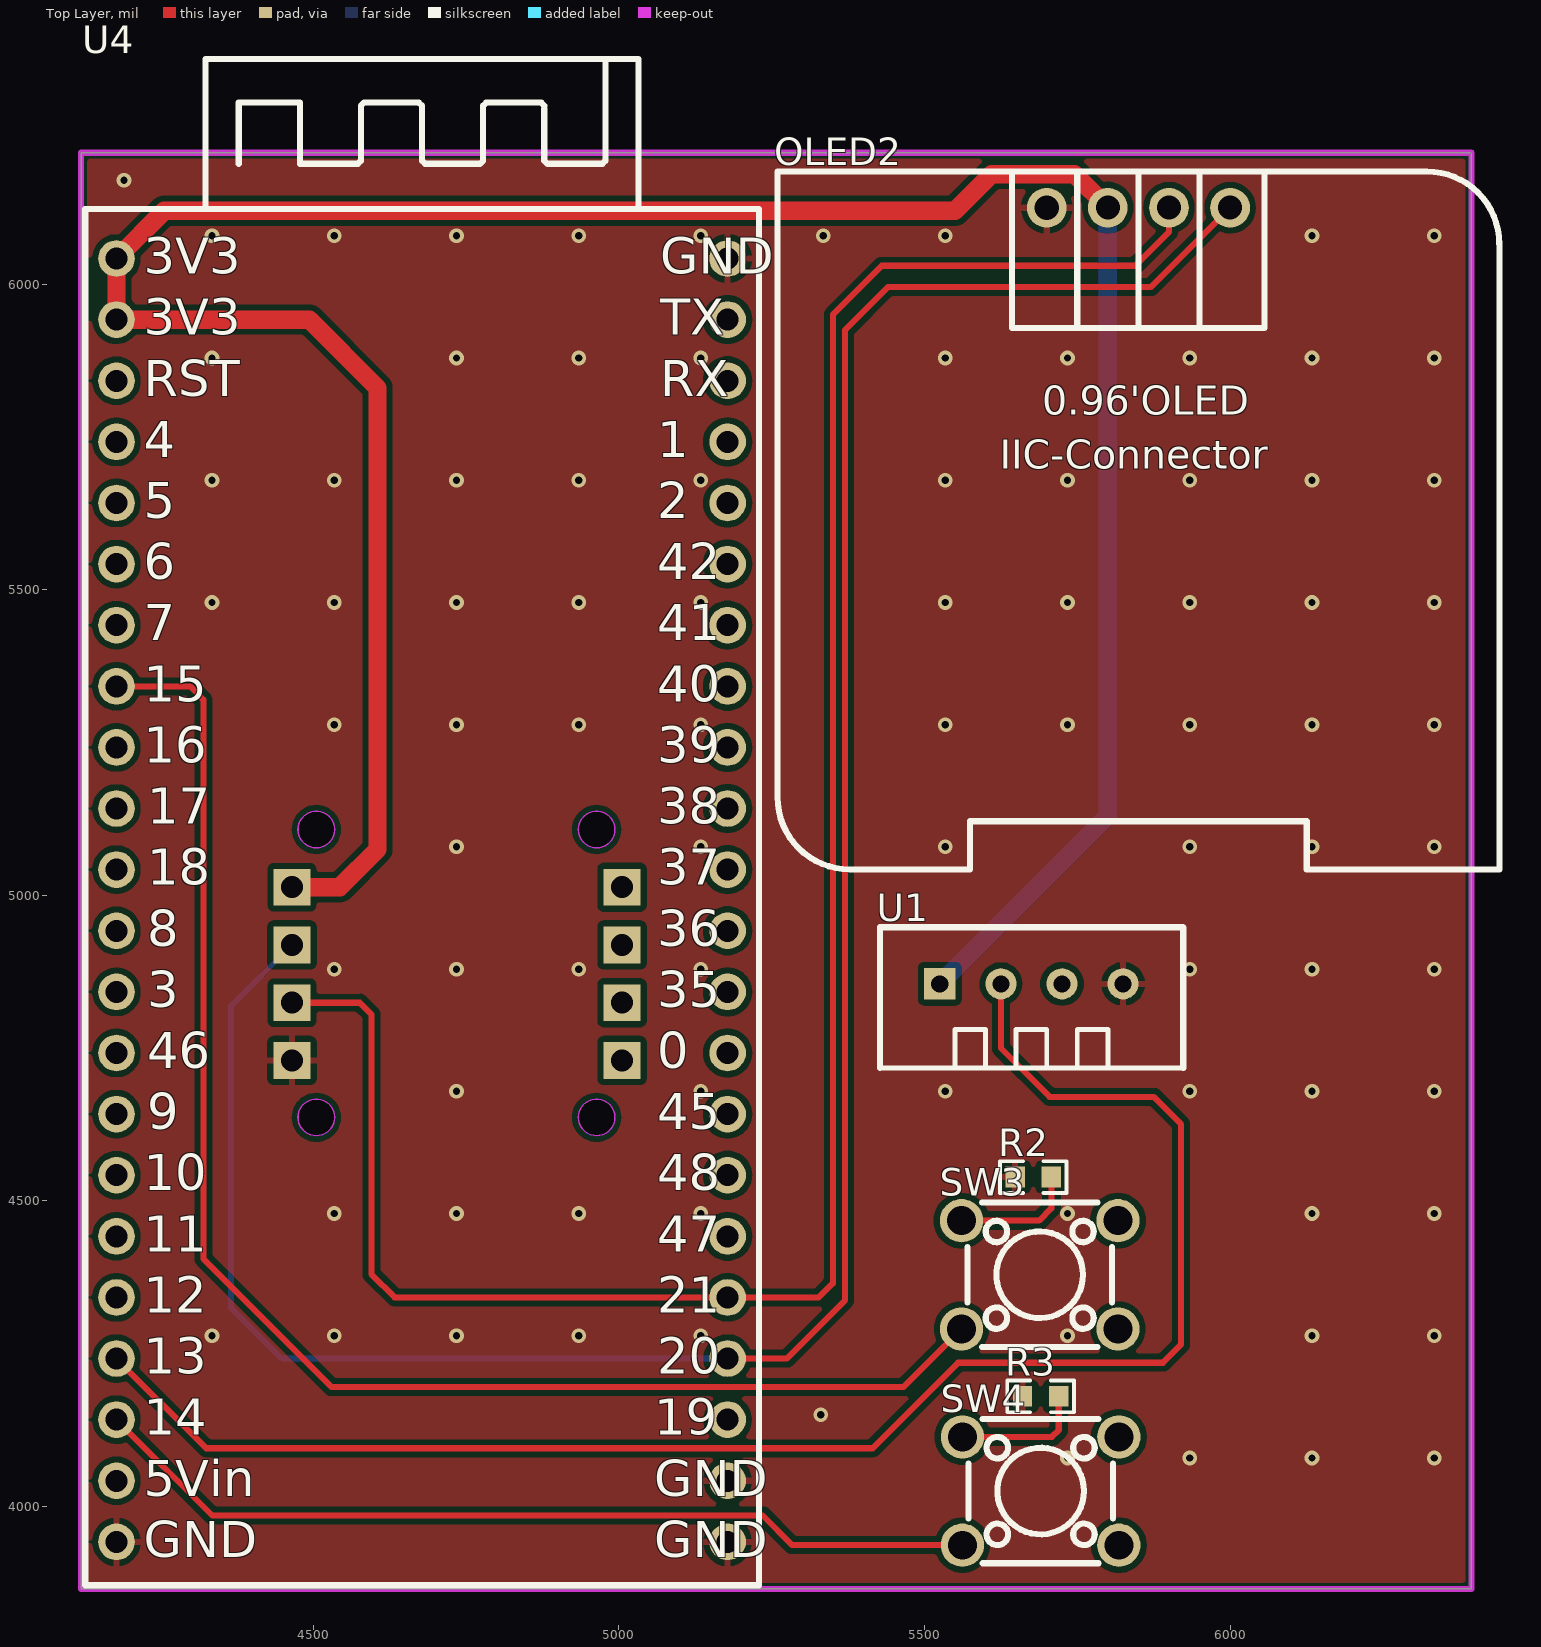
[diagram p0: Top Layer view]
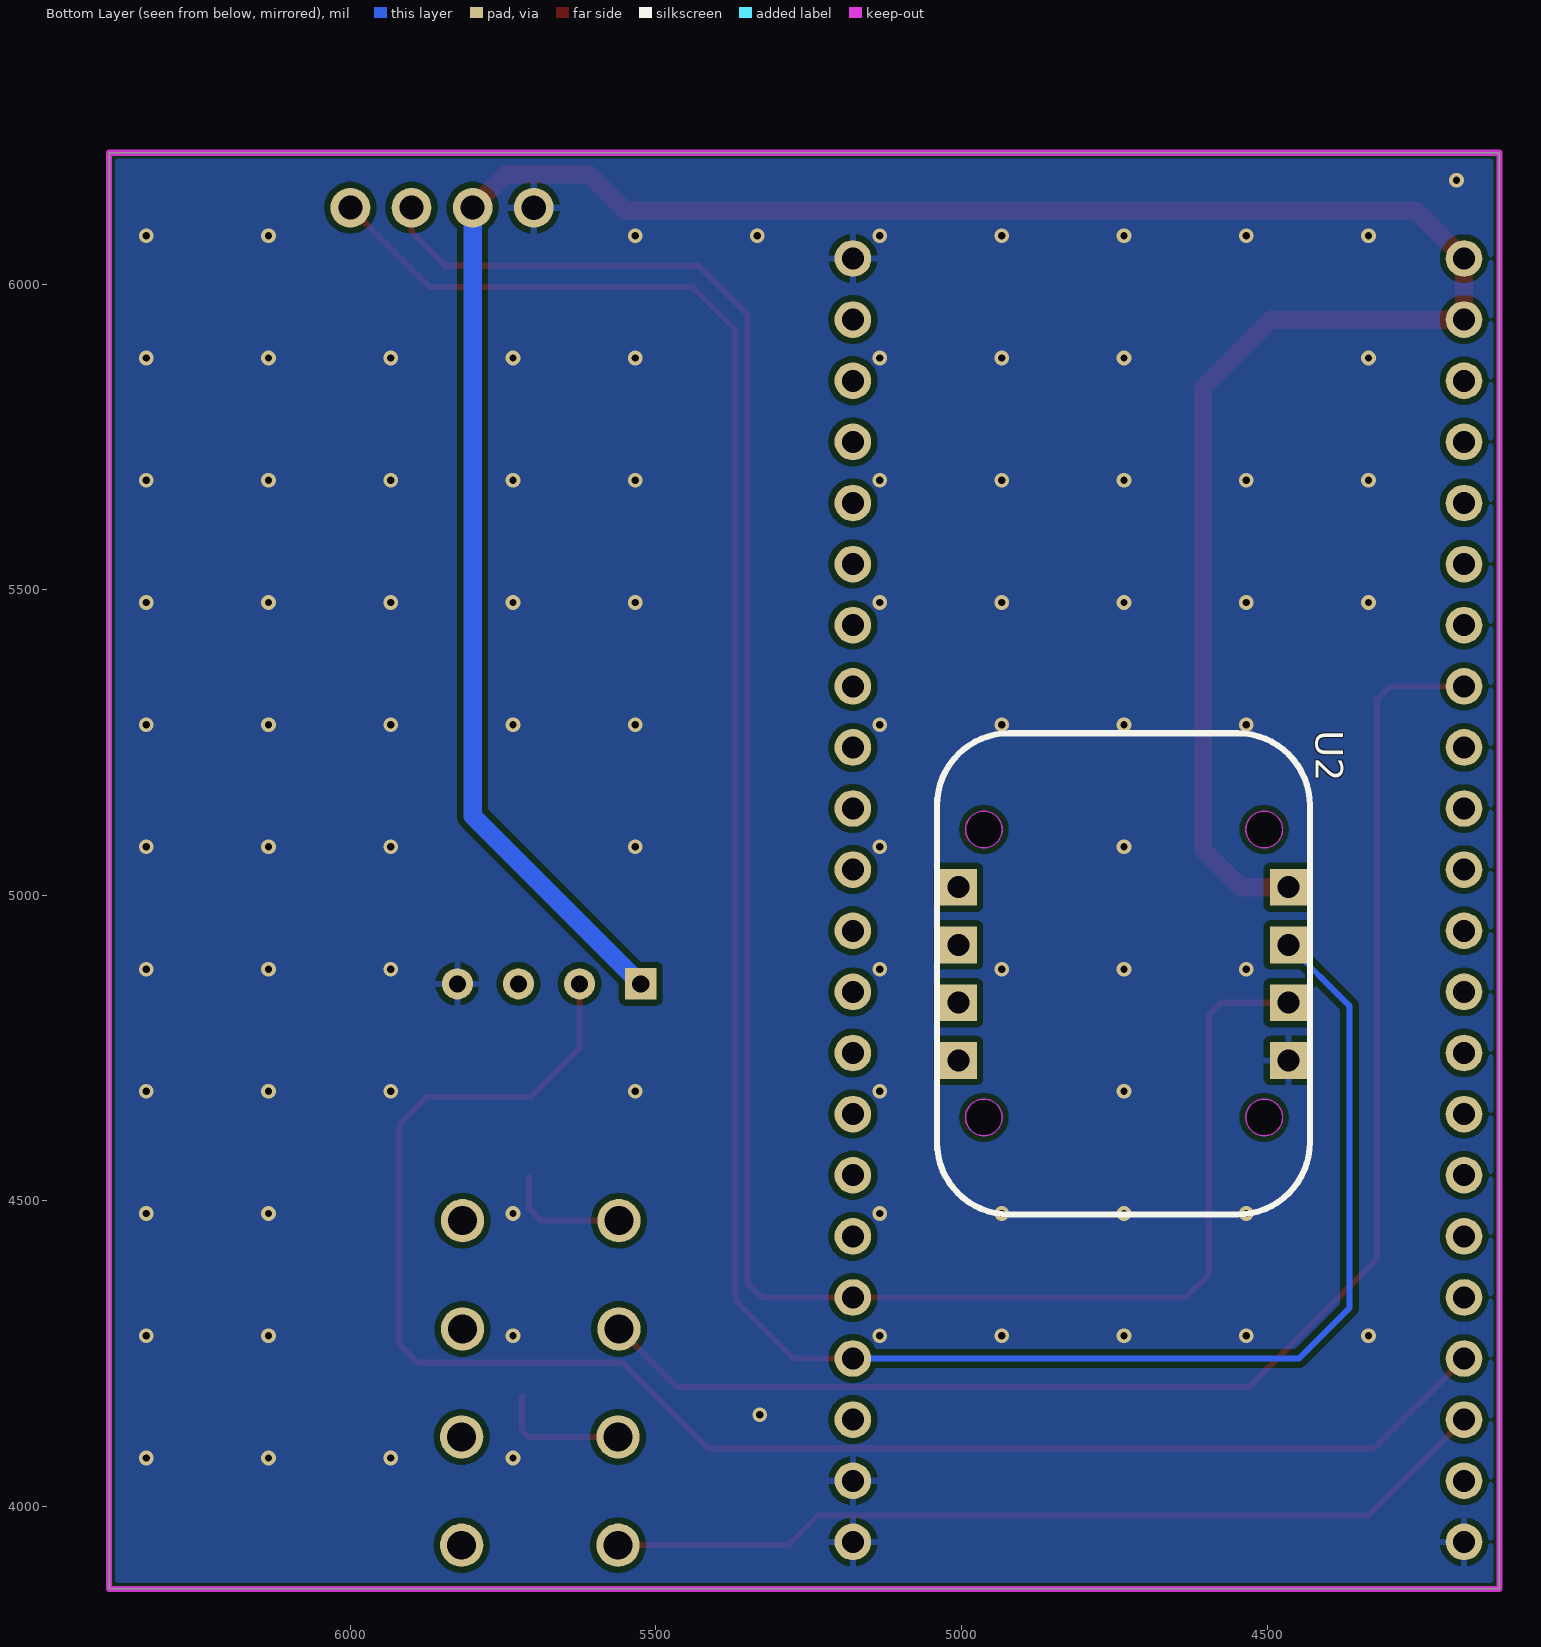
[diagram p1: Bottom Layer view, seen from below]
# Altium PCB MISC61243.pcbdoc
Units mil, origin at the board's own origin, x right, y up, seen from the top; angles counter-clockwise.
Board outline 2275 x 2350 mil, 2 copper layers (Top Layer, Bottom Layer), stack 62.206 mil thick; 8 components, 43 nets, 72 pads, 87 vias.

## Layer stack, top to bottom
Top Solder Mask Layer: solder mask 0.394, Dk 3.3
Top Layer: signal copper 1.379
Dielectric1: surface 59.449, FR4, Dk 4.5
Bottom Layer: signal copper 1.378
Bottom Solder Mask Layer: solder mask 0.394, Dk 3.3

## Board outline
4120,6215 4120,3865 6395,3865 6395,6215

## Design rules (kind name [scope] priority, off if disabled: settings)
BoardOutlineClearance copperThickness2oz_1 [All] p2 off: genericclearance=7.99 ignorepadtopadclearanceinfootprint=FALSE except(0: Arc-SplitContinuation Track-SplitContinuation SMDPad-SplitContinuation THPad-SplitContinuation Via-SplitContinuation Fill-SplitContinuation Region-SplitContinuation Poly-SplitContinuation Text-SplitContinuation Hole-SplitContinuation; 5.98: Arc-CutoutEdge Track-CutoutEdge SMDPad-CutoutEdge THPad-CutoutEdge Via-CutoutEdge Text-CutoutEdge; 6.9: Hole-OutlineEdge Hole-CutoutEdge; 10: Poly-OutlineEdge Poly-CutoutEdge; 11.81: Arc-OutlineEdge Track-OutlineEdge SMDPad-OutlineEdge THPad-OutlineEdge Via-OutlineEdge Fill-OutlineEdge Region-OutlineEdge Text-OutlineEdge Fill-CutoutEdge Region-CutoutEdge)
BoardOutlineClearance Plane_innerPlane_1 [All] p4 off: genericclearance=4.02 ignorepadtopadclearanceinfootprint=FALSE except(0: Arc-SplitContinuation Track-SplitContinuation SMDPad-SplitContinuation THPad-SplitContinuation Via-SplitContinuation Fill-SplitContinuation Region-SplitContinuation Poly-SplitContinuation Text-SplitContinuation Hole-SplitContinuation; 5.98: Arc-CutoutEdge Track-CutoutEdge SMDPad-CutoutEdge THPad-CutoutEdge Via-CutoutEdge Text-CutoutEdge; 6.9: Hole-OutlineEdge Hole-CutoutEdge; 10: Poly-OutlineEdge Poly-CutoutEdge; 11.81: Arc-OutlineEdge Track-OutlineEdge SMDPad-OutlineEdge THPad-OutlineEdge Via-OutlineEdge Fill-OutlineEdge Region-OutlineEdge Text-OutlineEdge Fill-CutoutEdge Region-CutoutEdge)
BoardOutlineClearance Copper_copperRegion_1 [All] p6 off: genericclearance=4.02 ignorepadtopadclearanceinfootprint=FALSE except(0: Arc-SplitContinuation Track-SplitContinuation SMDPad-SplitContinuation THPad-SplitContinuation Via-SplitContinuation Fill-SplitContinuation Region-SplitContinuation Poly-SplitContinuation Text-SplitContinuation Hole-SplitContinuation; 5.98: Arc-CutoutEdge Track-CutoutEdge SMDPad-CutoutEdge THPad-CutoutEdge Via-CutoutEdge Text-CutoutEdge; 6.9: Hole-OutlineEdge Hole-CutoutEdge; 10: Poly-OutlineEdge Poly-CutoutEdge; 11.81: Arc-OutlineEdge Track-OutlineEdge SMDPad-OutlineEdge THPad-OutlineEdge Via-OutlineEdge Fill-OutlineEdge Region-OutlineEdge Text-OutlineEdge Fill-CutoutEdge Region-CutoutEdge)
BoardOutlineClearance Copper_copperRegion_copperThickness1oz_1 [All] p8 off: genericclearance=4.02 ignorepadtopadclearanceinfootprint=FALSE except(0: Arc-SplitContinuation Track-SplitContinuation SMDPad-SplitContinuation THPad-SplitContinuation Via-SplitContinuation Fill-SplitContinuation Region-SplitContinuation Poly-SplitContinuation Text-SplitContinuation Hole-SplitContinuation; 5.98: Arc-CutoutEdge Track-CutoutEdge SMDPad-CutoutEdge THPad-CutoutEdge Via-CutoutEdge Text-CutoutEdge; 6.9: Hole-OutlineEdge Hole-CutoutEdge; 10: Poly-OutlineEdge Poly-CutoutEdge; 11.81: Arc-OutlineEdge Track-OutlineEdge SMDPad-OutlineEdge THPad-OutlineEdge Via-OutlineEdge Fill-OutlineEdge Region-OutlineEdge Text-OutlineEdge Fill-CutoutEdge Region-CutoutEdge)
BoardOutlineClearance Copper_copperRegion_Copper_copperRegion_1 [All] p10 off: genericclearance=4.02 ignorepadtopadclearanceinfootprint=FALSE except(0: Arc-SplitContinuation Track-SplitContinuation SMDPad-SplitContinuation THPad-SplitContinuation Via-SplitContinuation Fill-SplitContinuation Region-SplitContinuation Poly-SplitContinuation Text-SplitContinuation Hole-SplitContinuation; 5.98: Arc-CutoutEdge Track-CutoutEdge SMDPad-CutoutEdge THPad-CutoutEdge Via-CutoutEdge Text-CutoutEdge; 6.9: Hole-OutlineEdge Hole-CutoutEdge; 10: Poly-OutlineEdge Poly-CutoutEdge; 11.81: Arc-OutlineEdge Track-OutlineEdge SMDPad-OutlineEdge THPad-OutlineEdge Via-OutlineEdge Fill-OutlineEdge Region-OutlineEdge Text-OutlineEdge Fill-CutoutEdge Region-CutoutEdge)
BoardOutlineClearance copperThickness1oz_1 [All] p12: genericclearance=4.02 ignorepadtopadclearanceinfootprint=FALSE except(0: Arc-SplitContinuation Track-SplitContinuation SMDPad-SplitContinuation THPad-SplitContinuation Via-SplitContinuation Fill-SplitContinuation Region-SplitContinuation Poly-SplitContinuation Text-SplitContinuation Hole-SplitContinuation; 5.98: Arc-CutoutEdge Track-CutoutEdge SMDPad-CutoutEdge THPad-CutoutEdge Via-CutoutEdge Text-CutoutEdge; 6.9: Hole-OutlineEdge Hole-CutoutEdge; 10: Poly-OutlineEdge Poly-CutoutEdge; 11.81: Arc-OutlineEdge Track-OutlineEdge SMDPad-OutlineEdge THPad-OutlineEdge Via-OutlineEdge Fill-OutlineEdge Region-OutlineEdge Text-OutlineEdge Fill-CutoutEdge Region-CutoutEdge)
Clearance copperThickness2oz [All] p1 off: gap=7.99 ignorepadtopadclearanceinfootprint=FALSE except(5.98: SMDPad-Track SMDPad-SMDPad THPad-Track SMDPad-THPad THPad-THPad Track-Via SMDPad-Via THPad-Via Via-Via Fill-SMDPad Region-SMDPad Fill-THPad Region-THPad Fill-Via Region-Via Fill-Fill Fill-Region Region-Region Arc-Track Arc-SMDPad Arc-THPad Arc-Via Fill-Arc Region-Arc Arc-Arc Text-Track SMDPad-Text Text-THPad Text-Via Fill-Text Region-Text Arc-Text Text-Text; 6.9: Hole-Track Hole-SMDPad Hole-THPad Hole-Via Fill-Hole Region-Hole Hole-Arc Hole-Text; 10: Poly-Track Poly-SMDPad Poly-THPad Poly-Via Poly-Fill Poly-Region Poly-Poly Poly-Arc Poly-Text Poly-Hole; 11.81: Fill-Track Region-Track)
Clearance Plane_innerPlane [All] p3 off: gap=4.02 ignorepadtopadclearanceinfootprint=FALSE except(5.98: SMDPad-Track SMDPad-SMDPad THPad-Track SMDPad-THPad THPad-THPad Track-Via SMDPad-Via THPad-Via Via-Via Fill-SMDPad Region-SMDPad Fill-THPad Region-THPad Fill-Via Region-Via Fill-Fill Fill-Region Region-Region Arc-Track Arc-SMDPad Arc-THPad Arc-Via Fill-Arc Region-Arc Arc-Arc Text-Track SMDPad-Text Text-THPad Text-Via Fill-Text Region-Text Arc-Text Text-Text; 6.9: Hole-Track Hole-SMDPad Hole-THPad Hole-Via Fill-Hole Region-Hole Hole-Arc Hole-Text; 10: Poly-Track Poly-SMDPad Poly-THPad Poly-Via Poly-Fill Poly-Region Poly-Poly Poly-Arc Poly-Text Poly-Hole; 11.81: Fill-Track Region-Track)
Clearance Copper_copperRegion [All] p5 off: gap=4.02 ignorepadtopadclearanceinfootprint=FALSE except(5.98: SMDPad-Track SMDPad-SMDPad THPad-Track SMDPad-THPad THPad-THPad Track-Via SMDPad-Via THPad-Via Via-Via Fill-SMDPad Region-SMDPad Fill-THPad Region-THPad Fill-Via Region-Via Fill-Fill Fill-Region Region-Region Arc-Track Arc-SMDPad Arc-THPad Arc-Via Fill-Arc Region-Arc Arc-Arc Text-Track SMDPad-Text Text-THPad Text-Via Fill-Text Region-Text Arc-Text Text-Text; 6.9: Hole-Track Hole-SMDPad Hole-THPad Hole-Via Fill-Hole Region-Hole Hole-Arc Hole-Text; 10: Poly-Track Poly-SMDPad Poly-THPad Poly-Via Poly-Fill Poly-Region Poly-Poly Poly-Arc Poly-Text Poly-Hole; 11.81: Fill-Track Region-Track)
Clearance Copper_copperRegion_copperThickness1oz [All] p7 off: gap=4.02 ignorepadtopadclearanceinfootprint=FALSE except(5.98: SMDPad-Track SMDPad-SMDPad THPad-Track SMDPad-THPad THPad-THPad Track-Via SMDPad-Via THPad-Via Via-Via Fill-SMDPad Region-SMDPad Fill-THPad Region-THPad Fill-Via Region-Via Fill-Fill Fill-Region Region-Region Arc-Track Arc-SMDPad Arc-THPad Arc-Via Fill-Arc Region-Arc Arc-Arc Text-Track SMDPad-Text Text-THPad Text-Via Fill-Text Region-Text Arc-Text Text-Text; 6.9: Hole-Track Hole-SMDPad Hole-THPad Hole-Via Fill-Hole Region-Hole Hole-Arc Hole-Text; 10: Poly-Track Poly-SMDPad Poly-THPad Poly-Via Poly-Fill Poly-Region Poly-Poly Poly-Arc Poly-Text Poly-Hole; 11.81: Fill-Track Region-Track)
Clearance Copper_copperRegion_Copper_copperRegion [All] p9 off: gap=4.02 ignorepadtopadclearanceinfootprint=FALSE except(5.98: SMDPad-Track SMDPad-SMDPad THPad-Track SMDPad-THPad THPad-THPad Track-Via SMDPad-Via THPad-Via Via-Via Fill-SMDPad Region-SMDPad Fill-THPad Region-THPad Fill-Via Region-Via Fill-Fill Fill-Region Region-Region Arc-Track Arc-SMDPad Arc-THPad Arc-Via Fill-Arc Region-Arc Arc-Arc Text-Track SMDPad-Text Text-THPad Text-Via Fill-Text Region-Text Arc-Text Text-Text; 6.9: Hole-Track Hole-SMDPad Hole-THPad Hole-Via Fill-Hole Region-Hole Hole-Arc Hole-Text; 10: Poly-Track Poly-SMDPad Poly-THPad Poly-Via Poly-Fill Poly-Region Poly-Poly Poly-Arc Poly-Text Poly-Hole; 11.81: Fill-Track Region-Track)
Clearance copperThickness1oz [All] p11: gap=4.02 ignorepadtopadclearanceinfootprint=FALSE except(5.98: SMDPad-Track SMDPad-SMDPad THPad-Track SMDPad-THPad THPad-THPad Track-Via SMDPad-Via THPad-Via Via-Via Fill-SMDPad Region-SMDPad Fill-THPad Region-THPad Fill-Via Region-Via Fill-Fill Fill-Region Region-Region Arc-Track Arc-SMDPad Arc-THPad Arc-Via Fill-Arc Region-Arc Arc-Arc Text-Track SMDPad-Text Text-THPad Text-Via Fill-Text Region-Text Arc-Text Text-Text; 6.9: Hole-Track Hole-SMDPad Hole-THPad Hole-Via Fill-Hole Region-Hole Hole-Arc Hole-Text; 10: Poly-Track Poly-SMDPad Poly-THPad Poly-Via Poly-Fill Poly-Region Poly-Poly Poly-Arc Poly-Text Poly-Hole; 11.81: Fill-Track Region-Track)
DiffPairsRouting differentialPair [All] p1: maxlimit=6 minlimit=6 mostfreqgap=6 toplayer_minwidth=5 toplayer_prefwidth=10 toplayer_maxwidth=100 toplayer_mingap=6 toplayer_prefgap=6 toplayer_maxgap=6 bottomlayer_minwidth=5 bottomlayer_prefwidth=10 bottomlayer_maxwidth=100 bottomlayer_mingap=6 bottomlayer_prefgap=6 bottomlayer_maxgap=6 maxuncoupledlength=10
HoleToHoleClearance otherClearance [All] p1: gap=11.81 allowstackedmicrovias=TRUE
Length netLength [All] p1: minlimit=0 maxlimit=0
PasteMaskExpansion pasteMaskExpansion [All] p1: expansion=0
PlaneConnect innerPlane [All] p1: planeconnectstyle=Relief reliefexpansion=20 reliefentries=4 reliefconductorwidth=10 reliefairgap=10
PolygonConnect copperRegion_copperThickness1oz [All] p1 off: connectstyle=Relief reliefconductorwidth=10 reliefentries=4 polygonreliefangle="90 Angle" airgapwidth=10 via.connectstyle=Relief via.reliefconductorwidth=10 via.reliefentries=4 via.polygonreliefangle="90 Angle" via.airgapwidth=10
PolygonConnect copperRegion_Copper_copperRegion [All] p2 off: connectstyle=Relief reliefconductorwidth=10 reliefentries=4 polygonreliefangle="90 Angle" airgapwidth=10 via.connectstyle=Relief via.reliefconductorwidth=10 via.reliefentries=4 via.polygonreliefangle="90 Angle" via.airgapwidth=10
PolygonConnect copperRegion [All] p3: connectstyle=Relief reliefconductorwidth=10 reliefentries=4 polygonreliefangle="90 Angle" airgapwidth=10 via.connectstyle=Relief via.reliefconductorwidth=10 via.reliefentries=4 via.polygonreliefangle="90 Angle" via.airgapwidth=10
RoutingVias viaSize [All] p1: holewidth=12.01 width=24.02 viastyle="Through Hole" minholewidth=11.81 minwidth=19.68 maxholewidth=248.03 maxwidth=393.7
SolderMaskExpansion solderMaskExpansion [IsVia] p1: expansion=-1000 istentingtop=TRUE
SolderMaskExpansion solderMaskExpansion [All] p2: expansion=2 istentingtop=FALSE
Width copperThickness2oz_2 [All] p1 off: maxlimit=100 minlimit=8 preferedwidth=10
Width copperThickness1oz_2 [All] p2: maxlimit=100 minlimit=5 preferedwidth=10

## Components (designator, comment, footprint, x,y, rotation, side; value= is the part's Value field where it differs from the comment)
OLED2 "" 0.96OLED_4P 5850,6125 r0 top
R2 "10K" R0603 5677.93,4538.85 r0 top
R3 "10K" R0603 5690,4180 r0 top
SW3 "" SW-TH_4P-L6.0-W6.0-P4.50-LS6.5 5688.53,4378.85 r0 top
SW4 "" SW-TH_4P-L6.0-W6.0-P4.50-LS6.5 5690,4025 r0 top
U1 "DHT11" SENSOR-TH_DHT11 5675,4855 r0 top
U2 "MAX30102" MAX30102 4430,5265 r270 bottom
U4 "NO" ESP32S3 4677.78,4996.83 r0 top

## Footprints (in the part's own frame and the unit in brackets; to place one, negate y for a bottom-side part, rotate by r counter-clockwise, add the part's x,y. Pads: shape width x height; smd on the part's side, far side on the other; paste and mask are expansions set on the pad)
0.96OLED_4P [mm]
  round 1.65 hole 1 copper offset 0,0: 1(-3.81,-0.001) 2(-1.27,0.002) 3(1.27,0.002) 4(3.81,0.002)
  silkscreen extent -15,-27.5 15,1.5
ESP32S3 [mil]
  round 60 hole 36: 1(-500,-1055) 2(-500,-955) 3(-500,-855) 4(-500,-755) 5(-500,-655) 6(-500,-555) 7(-500,-455) 8(-500,-355) 9(-500,-255) 10(-500,-155) 11(-500,-55) 12(-500,45) 13(-500,145) 14(-500,245) 15(-500,345) 16(-500,445) 17(-500,545) 18(-500,645) 19(-500,745) 20(-500,845) 21(-500,945) 22(-500,1045) 23(500,-1055) 24(500,-955) 25(500,-855) 26(500,-755) 27(500,-655) 28(500,-555) 29(500,-455) 30(500,-355) 31(500,-255) 32(500,-155) 33(500,-55) 34(500,45) 35(500,145) 36(500,245) 37(500,345) 38(500,445) 39(500,545) 40(500,645) 41(500,745) 42(500,845) 43(500,945) 44(500,1045)
  silkscreen extent -551,-1126 551,1371
MAX30102 [mil]
  rect 60x60 hole 36: 1(251.97,-35) 2(346.46,-35) 3(440.94,-35) 4(535.43,-35) 5(251.97,-575) 6(346.46,-575) 7(440.94,-575) 8(535.43,-575)
  Board Outline Layer circle w0.1: c157.48,-74.8 r30
  Board Outline Layer circle w0.1: c157.48,-533.46 r30
  Board Outline Layer circle w0.1: c628.5,-74.8 r30
  Board Outline Layer circle w0.1: c628.5,-533.46 r30
  Board Outline Layer region: 157.48,-104.8 170.5,-101.83 180.94,-93.51 186.73,-81.48 186.73,-68.13 180.94,-56.1 170.5,-47.77 157.48,-44.8 157.48,-44.8 144.46,-47.77 134.03,-56.1 128.23,-68.13 128.23,-81.48 134.03,-93.51 144.46,-101.83 157.48,-104.8
  Board Outline Layer region: 157.48,-104.8 162.17,-104.43 166.75,-103.33 171.1,-101.53 175.11,-99.07 178.69,-96.02 181.75,-92.44 184.21,-88.42 186.01,-84.07 187.11,-79.5 187.48,-74.8 187.11,-70.11 186.01,-65.53 184.21,-61.18 181.75,-57.17 178.69,-53.59 175.11,-50.53 171.1,-48.07 166.75,-46.27 162.17,-45.17 157.48,-44.8 152.79,-45.17 148.21,-46.27 143.86,-48.07 139.85,-50.53 136.27,-53.59 133.21,-57.17 130.75,-61.18 128.95,-65.53 127.85,-70.11 127.48,-74.8 127.85,-79.5 128.95,-84.07 130.75,-88.42 133.21,-92.44 136.27,-96.02 139.85,-99.07 143.86,-101.53 148.21,-103.33 152.79,-104.43
  Board Outline Layer region: 157.48,-563.46 170.5,-560.49 180.94,-552.17 186.73,-540.14 186.73,-526.79 180.94,-514.76 170.5,-506.44 157.48,-503.46 157.48,-503.46 144.46,-506.44 134.03,-514.76 128.23,-526.79 128.23,-540.14 134.03,-552.17 144.46,-560.49 157.48,-563.46
  Board Outline Layer region: 157.48,-563.46 162.17,-563.1 166.75,-562 171.1,-560.19 175.11,-557.74 178.69,-554.68 181.75,-551.1 184.21,-547.08 186.01,-542.74 187.11,-538.16 187.48,-533.46 187.11,-528.77 186.01,-524.19 184.21,-519.84 181.75,-515.83 178.69,-512.25 175.11,-509.19 171.1,-506.73 166.75,-504.93 162.17,-503.83 157.48,-503.46 152.79,-503.83 148.21,-504.93 143.86,-506.73 139.85,-509.19 136.27,-512.25 133.21,-515.83 130.75,-519.84 128.95,-524.19 127.85,-528.77 127.48,-533.46 127.85,-538.16 128.95,-542.74 130.75,-547.08 133.21,-551.1 136.27,-554.68 139.85,-557.74 143.86,-560.19 148.21,-562 152.79,-563.1
  Board Outline Layer region: 628.5,-104.8 641.52,-101.83 651.96,-93.51 657.75,-81.48 657.75,-68.13 651.96,-56.1 641.52,-47.77 628.5,-44.8 628.5,-44.8 615.49,-47.77 605.05,-56.1 599.26,-68.13 599.26,-81.48 605.05,-93.51 615.49,-101.83 628.5,-104.8
  Board Outline Layer region: 628.5,-104.8 633.2,-104.43 637.77,-103.33 642.12,-101.53 646.14,-99.07 649.72,-96.02 652.77,-92.44 655.23,-88.42 657.04,-84.07 658.13,-79.5 658.5,-74.8 658.13,-70.11 657.04,-65.53 655.23,-61.18 652.77,-57.17 649.72,-53.59 646.14,-50.53 642.12,-48.07 637.77,-46.27 633.2,-45.17 628.5,-44.8 623.81,-45.17 619.23,-46.27 614.88,-48.07 610.87,-50.53 607.29,-53.59 604.23,-57.17 601.77,-61.18 599.97,-65.53 598.87,-70.11 598.5,-74.8 598.87,-79.5 599.97,-84.07 601.77,-88.42 604.23,-92.44 607.29,-96.02 610.87,-99.07 614.88,-101.53 619.23,-103.33 623.81,-104.43
  Board Outline Layer region: 628.5,-563.46 641.52,-560.49 651.96,-552.17 657.75,-540.14 657.75,-526.79 651.96,-514.76 641.52,-506.44 628.5,-503.46 628.5,-503.46 615.49,-506.44 605.05,-514.76 599.26,-526.79 599.26,-540.14 605.05,-552.17 615.49,-560.49 628.5,-563.46
  Board Outline Layer region: 628.5,-563.46 633.2,-563.1 637.77,-562 642.12,-560.19 646.14,-557.74 649.72,-554.68 652.77,-551.1 655.23,-547.08 657.04,-542.74 658.13,-538.16 658.5,-533.46 658.13,-528.77 657.04,-524.19 655.23,-519.84 652.77,-515.83 649.72,-512.25 646.14,-509.19 642.12,-506.73 637.77,-504.93 633.2,-503.83 628.5,-503.46 623.81,-503.83 619.23,-504.93 614.88,-506.73 610.87,-509.19 607.29,-512.25 604.23,-515.83 601.77,-519.84 599.97,-524.19 598.87,-528.77 598.5,-533.46 598.87,-538.16 599.97,-542.74 601.77,-547.08 604.23,-551.1 607.29,-554.68 610.87,-557.74 614.88,-560.19 619.23,-562 623.81,-563.1
  Multi-Layer board cut-out: 157.48,-104.8 170.5,-101.83 180.94,-93.51 186.73,-81.48 186.73,-68.13 180.94,-56.1 170.5,-47.77 157.48,-44.8 157.48,-44.8 144.46,-47.77 134.03,-56.1 128.23,-68.13 128.23,-81.48 134.03,-93.51 144.46,-101.83 157.48,-104.8
  Multi-Layer board cut-out: 157.48,-563.46 170.5,-560.49 180.94,-552.17 186.73,-540.14 186.73,-526.79 180.94,-514.76 170.5,-506.44 157.48,-503.46 157.48,-503.46 144.46,-506.44 134.03,-514.76 128.23,-526.79 128.23,-540.14 134.03,-552.17 144.46,-560.49 157.48,-563.46
  Multi-Layer board cut-out: 628.5,-104.8 641.52,-101.83 651.96,-93.51 657.75,-81.48 657.75,-68.13 651.96,-56.1 641.52,-47.77 628.5,-44.8 628.5,-44.8 615.49,-47.77 605.05,-56.1 599.26,-68.13 599.26,-81.48 605.05,-93.51 615.49,-101.83 628.5,-104.8
  Multi-Layer board cut-out: 628.5,-563.46 641.52,-560.49 651.96,-552.17 657.75,-540.14 657.75,-526.79 651.96,-514.76 641.52,-506.44 628.5,-503.46 628.5,-503.46 615.49,-506.44 605.05,-514.76 599.26,-526.79 599.26,-540.14 605.05,-552.17 615.49,-560.49 628.5,-563.46
  silkscreen extent 0,-610 787,0
R0603 [mil]
  rect 31.75x34.02 smd paste-3937.01 mask+2: 1(-29.66,0) 2(29.66,0)
  silkscreen extent -55,-26 55,26
SENSOR-TH_DHT11 [mil]
  rect 51x51 hole 28: 1(-150,0)
  round 51 hole 28: 2(-50,0) 3(50,0) 4(150,0)
  silkscreen extent -248,-138 248,93
SW-TH_4P-L6.0-W6.0-P4.50-LS6.5 [mm]
  round 1.8 hole 1.2: 1(-3.25,2.25) 2(3.25,2.25) 3(-3.25,-2.25) 4(3.25,-2.25)
  silkscreen extent -3,-3 3,3

## Via types
v1: diameter 24.02, hole 12, Top Layer to Bottom Layer, 87 vias

## Nets (pads, with @x,y where several pads share a name; then routed paths per layer and width w, separated by ;. In a path a pad name is that pad's centre, name@x,y a point inside that pad or via, vN(x,y) a via of type N, cw(c..) or ccw(c..) an arc to the next point about the centre after c; other vN are vias at no path point)
0: U4.31
1: U4.41
2: U4.40
3: U4.10
4: U4.19
5: U4.18
6: U4.17
7: U4.16
8: U4.11
9: U4.8
10: U4.7
11: U4.6
12: U4.5
13: U1.2 U4.4 | length 2685.2
  Top Layer w10: U4.4 4324.61,4095 5415,4095 5555,4235 5890,4235 5920,4265 5920,4625 5875,4670 5705,4670 5625,4750 U1.2
14: SW4.3 U4.3 | length 1469.4
  Top Layer w10: U4.3 4334.61,3985 5235,3985 5283.58,3936.42 SW4.3
15: SW3.3 U4.15 | length 2433.3
  Top Layer w10: U4.15 4298.17,5341.83 4320,5320 4320,4405 4530,4195 5465.31,4195 SW3.3
16: U4.14
17: U4.13
18: U4.12
19: U4.25
20: OLED2.4 U2.2 U4.26 | length 4014.4
  Top Layer w10: U4.26 5274.31,4241.83 5370,4337.52 5370,5925 5440,5995 5869.95,5995 OLED2.4@6000,6125.05
  Bottom Layer w10: U2.2 4365,4818.54 4365,4325 4448.17,4241.83 U4.26
21: OLED2.3 U2.3 U4.27 | length 3574.3
  Top Layer w10: U2.3 4575.94,4824.06 4595,4805 4595,4380 4633.17,4341.83 U4.27 5326.83,4341.83 5350,4365 5350,5950 5430,6030 5845,6030 5900,6085 OLED2.3@5900,6125.05
35: U4.32
36: U4.33
37: U4.34
38: U4.35
39: U4.36
40: U4.37
41: U4.38
42: U4.39
45: U4.30
46: U4.9
47: U4.28
48: U4.29
$1N17208: R2.2 SW3.1 | length 206.6
  Top Layer w10: SW3.1 5687.43,4467.43 5707.59,4487.59 R2.2
$1N17209: R3.2 SW4.1 | length 217.5
  Top Layer w10: SW4.1 5708.58,4113.58 5719.66,4124.66 R3.2
+5V: U4.2
GND: OLED2.1 R2.1 R3.1 U1.4 U2.4 U4.1 U4.23 U4.24 U4.44
  other v1: 5734.1,4079.1 5934.1,4079.1 6134.1,4079.1 6334.1,4079.1 5330,4150 4334.1,4279.1 4534.1,4279.1 4734.1,4279.1 4934.1,4279.1 5134.1,4279.1 5734.1,4279.1 6134.1,4279.1 6334.1,4279.1 4534.1,4479.1 4734.1,4479.1 4934.1,4479.1 5134.1,4479.1 5734.1,4479.1 6134.1,4479.1 6334.1,4479.1 4734.1,4679.1 5134.1,4679.1 5534.1,4679.1 5934.1,4679.1 6134.1,4679.1 6334.1,4679.1 4534.1,4879.1 4734.1,4879.1 4934.1,4879.1 5134.1,4879.1 5934.1,4879.1 6134.1,4879.1 6334.1,4879.1 4734.1,5079.1 5134.1,5079.1 5534.1,5079.1 5934.1,5079.1 6134.1,5079.1 6334.1,5079.1 4534.1,5279.1 4734.1,5279.1 4934.1,5279.1 5134.1,5279.1 5534.1,5279.1 5734.1,5279.1 5934.1,5279.1 6134.1,5279.1 6334.1,5279.1 4334.1,5479.1 4534.1,5479.1 4734.1,5479.1 4934.1,5479.1 5134.1,5479.1 5534.1,5479.1 5734.1,5479.1 5934.1,5479.1 6134.1,5479.1 6334.1,5479.1 4334.1,5679.1 4534.1,5679.1 4734.1,5679.1 4934.1,5679.1 5134.1,5679.1 5534.1,5679.1 5734.1,5679.1 5934.1,5679.1 6134.1,5679.1 6334.1,5679.1 4334.1,5879.1 4734.1,5879.1 4934.1,5879.1 5134.1,5879.1 5534.1,5879.1 5734.1,5879.1 5934.1,5879.1 6134.1,5879.1 6334.1,5879.1 4334.1,6079.1 4534.1,6079.1 4734.1,6079.1 4934.1,6079.1 5134.1,6079.1 5334.1,6079.1 5534.1,6079.1 6134.1,6079.1 6334.1,6079.1 4190,6170
IO21: U2.8
RST: U4.20
RX: U4.42
TX: U4.43
VCC: OLED2.2 U1.1 U2.1 U4.21 U4.22 | length 4580.3
  Top Layer w30: U2.1 4543.03,5013.03 4605,5075 4605,5830 4493.17,5941.83 U4.21 U4.22 4255.95,6120 5550,6120 5610,6180 5745,6180 ; 5745.05,6180 OLED2.2@5800,6125.05
  Bottom Layer w30: U1.1 5800,5130 OLED2.2@5800,6125.05
pads on no net: SW3.2 SW3.4 SW4.2 SW4.4 U1.3 U2.5 U2.6 U2.7

## Polygon pours and split planes (outlines as drawn)
GND on Bottom Layer (solid, remove dead copper, pour order 2): 3525,7245 3525,3080 7700,3080 7700,7245
GND on Top Layer (solid, remove dead copper, pour order 2): 3000,7415 3000,3000 7930,3000 7930,7415

## Keep-outs
Board Outline Layer:
  the board outline again, w10